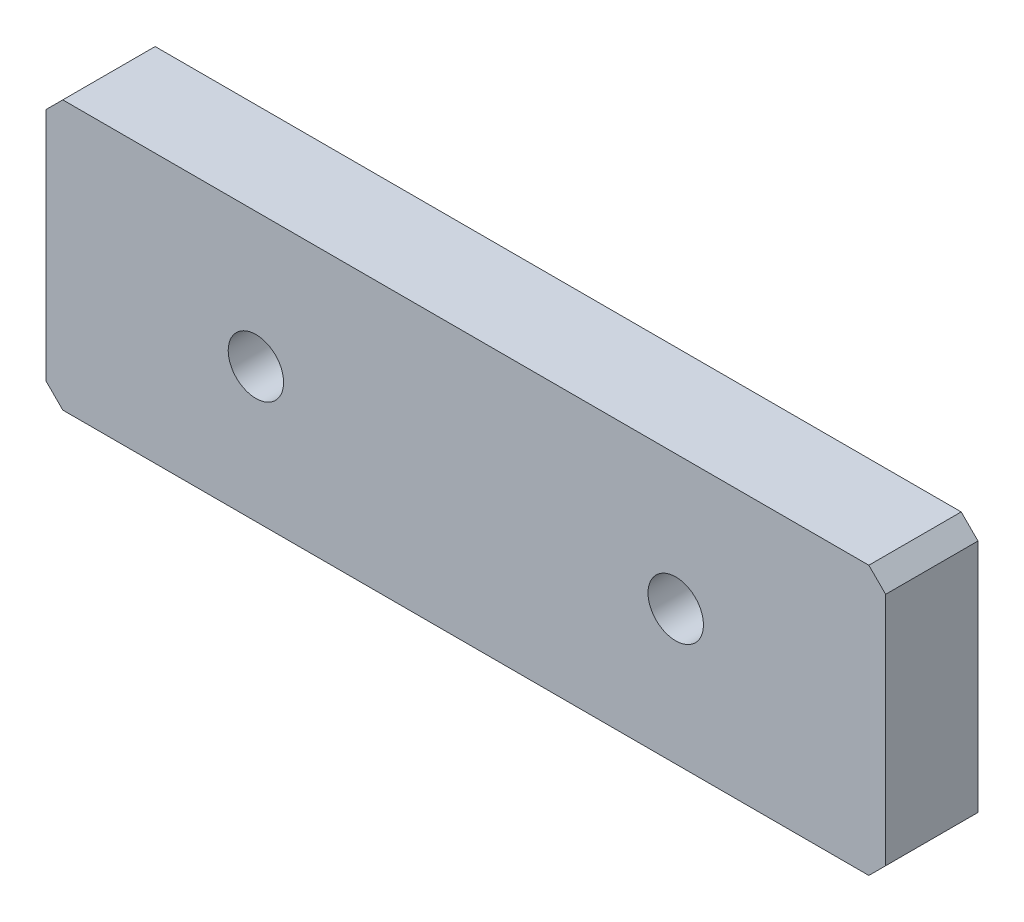
from build123d import *

# Parameters (mm, degrees)
SKETCH_1_W         = 50
SKETCH_1_H         = 16
EXTRUDE_1_DEPTH    = 2.75
HOLE_WIZARD_M4_1_D = 3.3
CHAMFER_1_SIZE     = 1


with BuildPart() as part:
    # 草图1 → 凸台-拉伸1 (new, symmetric)
    with BuildSketch(Plane.XY):
        Rectangle(SKETCH_1_W, SKETCH_1_H)
    extrude(amount=EXTRUDE_1_DEPTH, both=True)

    # M4 螺纹孔1 (through all)
    with Locations(Plane(origin=(0, 0, -2.75), x_dir=(-1, 0, 0), z_dir=(0, 0, -1))):
        with Locations((12.5, 0), (-12.5, 0)):
            Hole(HOLE_WIZARD_M4_1_D / 2)

    # 倒角1
    chamfer_1_edges = [part.edges().sort_by_distance(p)[0] for p in [
        (25, -8, 0),
        (-25, -8, 0),
        (-25, 8, 0),
        (25, 8, 0),
    ]]
    chamfer(chamfer_1_edges, length=CHAMFER_1_SIZE)


solid = part.part
